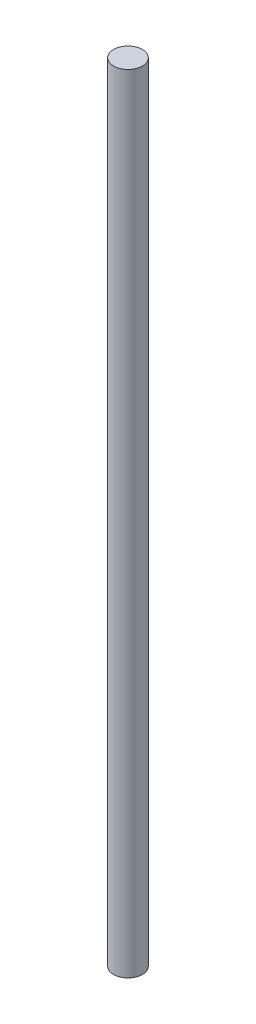
SolidWorks part; units mm, degrees
material "20#"
ref_plane "Front Plane" through (0, 0, 0) normal (0, 0, 1) x (1, 0, 0)
ref_plane "Top Plane" through (0, 0, 0) normal (0, 1, 0) x (1, 0, 0)
ref_plane "Right Plane" through (0, 0, 0) normal (1, 0, 0) x (0, 0, -1)
sketch "Sketch1" plane through (0, 0, 0) normal (0, 1, 0) x (1, 0, 0)
  circle A0 centre (0, 0) radius 1.5
  dimension "D1" = 3
extrude "Boss-Extrude1" add sketch "Sketch1" along normal blind 82
